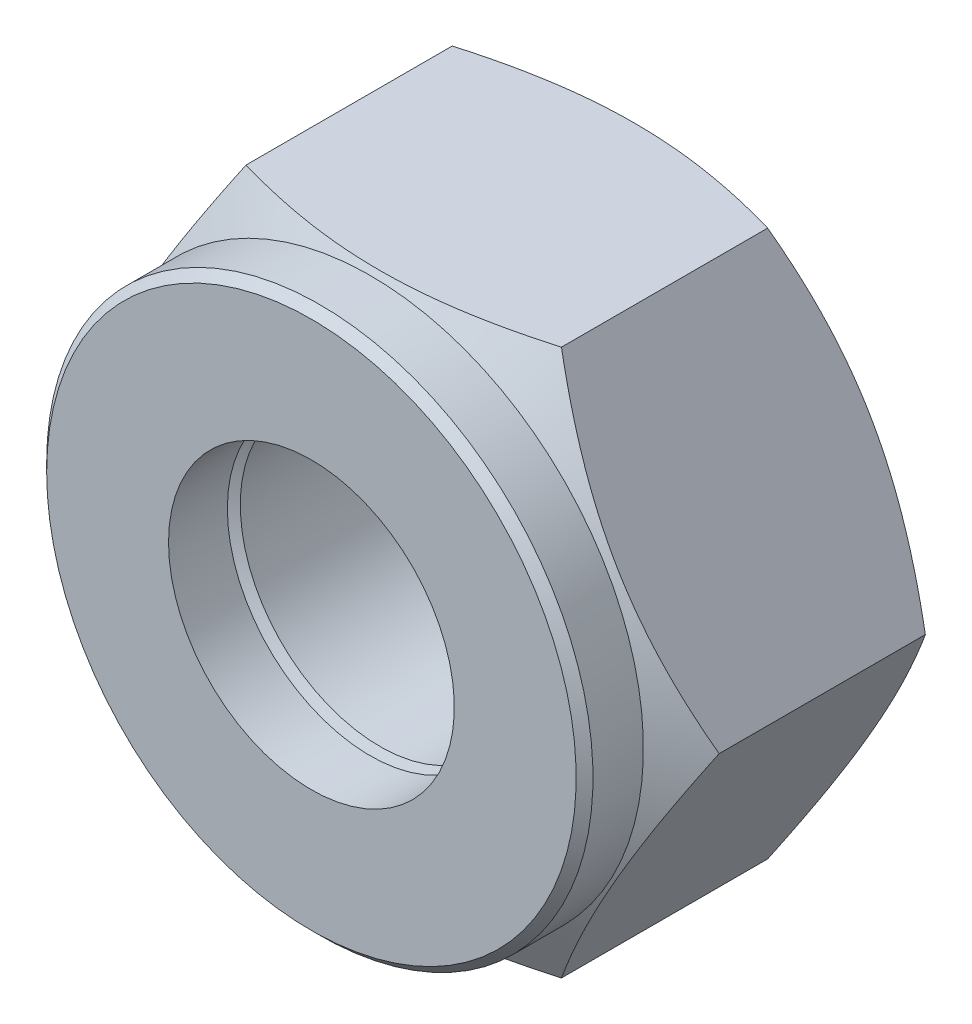
SolidWorks part; units mm, degrees
ref_plane "Front" through (0, 0, 0) normal (0, 0, 1) x (1, 0, 0)
ref_plane "Top" through (0, 0, 0) normal (0, 1, 0) x (1, 0, 0)
ref_plane "Right" through (0, 0, 0) normal (1, 0, 0) x (0, 0, -1)
sketch "Sketch1" plane through (0, 0, 0) normal (0, 0, 1) x (1, 0, 0)
  line L1 (3.7528, -6.5) -> (7.5056, 0)
  line L2 (7.5056, 0) -> (3.7528, 6.5)
  line L3 (3.7528, 6.5) -> (-3.7528, 6.5)
  line L4 (-3.7528, 6.5) -> (-7.5056, 0)
  line L5 (-7.5056, 0) -> (-3.7528, -6.5)
  line L6 (-3.7528, -6.5) -> (3.7528, -6.5)
  circle A0 centre (0, 0) radius 6.5 construction
  circle A1 centre (0, 0) radius 3.3235
  dimension "D" = 6.647
  dimension "s" = 13
extrude "BaseNut" add sketch "Sketch1" against normal blind 6.5
cosmetic thread "ThreadCosmetic1" parameters "D"=8
sketch "Sketch2" plane through (0, 0, 0) normal (0, 1, 0) x (1, 0, 0)
  line L0 (-7.5056, 6.5) -> (-6.125, 6.5)
  line L2 (-6.125, 6.5) -> (-7.5056, 5.7029)
  line L3 (-7.5056, 5.7029) -> (-7.5056, 6.5)
  line L4 (0, 3.3759) -> (0, -9.8171) construction
  line L6 (-9.7712, 3.25) -> (9.8853, 3.25) construction
  line L7 (-7.5056, 0.7971) -> (-7.5056, 0)
  line L8 (-6.125, 0) -> (-7.5056, 0.7971)
  line L9 (-7.5056, 0) -> (-6.125, 0)
  dimension "D1" = 30
  dimension "dw" = 12.25
  dimension "D2" = 3.25
revolve "Double-Chamfer" cut sketch "Sketch2" angle 360 about L4
chamfer "EndChamfer" distance 0.4 angle 30 2 edges at (3.3235, 0, -6.5) (3.3235, 0, 0)
sketch "Sketch3" plane through (0, 0, 0) normal (0, 1, 0) x (1, 0, 0)
  line L0 (0, 6.7075) -> (0, -2.1252) construction
  line L1 (2.647, 6.4383) -> (3.3235, 6.4383)
  line L2 (3.3235, 6.4383) -> (3.9094, 6.1)
  line L3 (3.9094, 6.1) -> (3.3235, 5.7618)
  line L4 (3.3235, 5.7618) -> (2.647, 5.7618)
  line L5 (2.647, 5.7618) -> (2.647, 6.4383)
  line L6 (3.3235, 6.1) -> (-3.3235, 6.1) construction
  dimension "D1" = 0.6765
  dimension "D2" = 6.647
revolve "Cut-Revolve10" [suppressed] cut sketch "Sketch3" angle 360 about L0
pattern_linear "LPattern10" [suppressed] count 4 spacing 0.8118 along (0, 0, 1)
sketch "草图1" plane through (0, 0, 0) normal (0, 0, 1) x (1, 0, 0)
  circle A0 centre (0, 0) radius 6.5
  circle A1 centre (0, 0) radius 3.4
  dimension "D1" = 6.8
extrude "凸台-拉伸1" add sketch "草图1" along normal blind 1.4
chamfer "倒角1" distance 0.2 angle 45 1 edges at (6.5, 0, 1.4)
equation "\"dw@Sketch2\" = \"s@Sketch1\"-0.75"
equation "\"D1@EndChamfer\" = \"m@BaseNut\" / 10"
equation "\"D2@Sketch3\" = \"D@Sketch1\""
equation "\"D1@Sketch3\" = (  \"D@ThreadCosmetic1\" - \"D@Sketch1\" )  / 2"
equation "\"D3@LPattern10\" = \"D1@Sketch3\" * 1.2"
equation "\"D1@LPattern10\" = (  \"m@BaseNut\" - \"D1@EndChamfer\" )  / \"D3@LPattern10\" "
